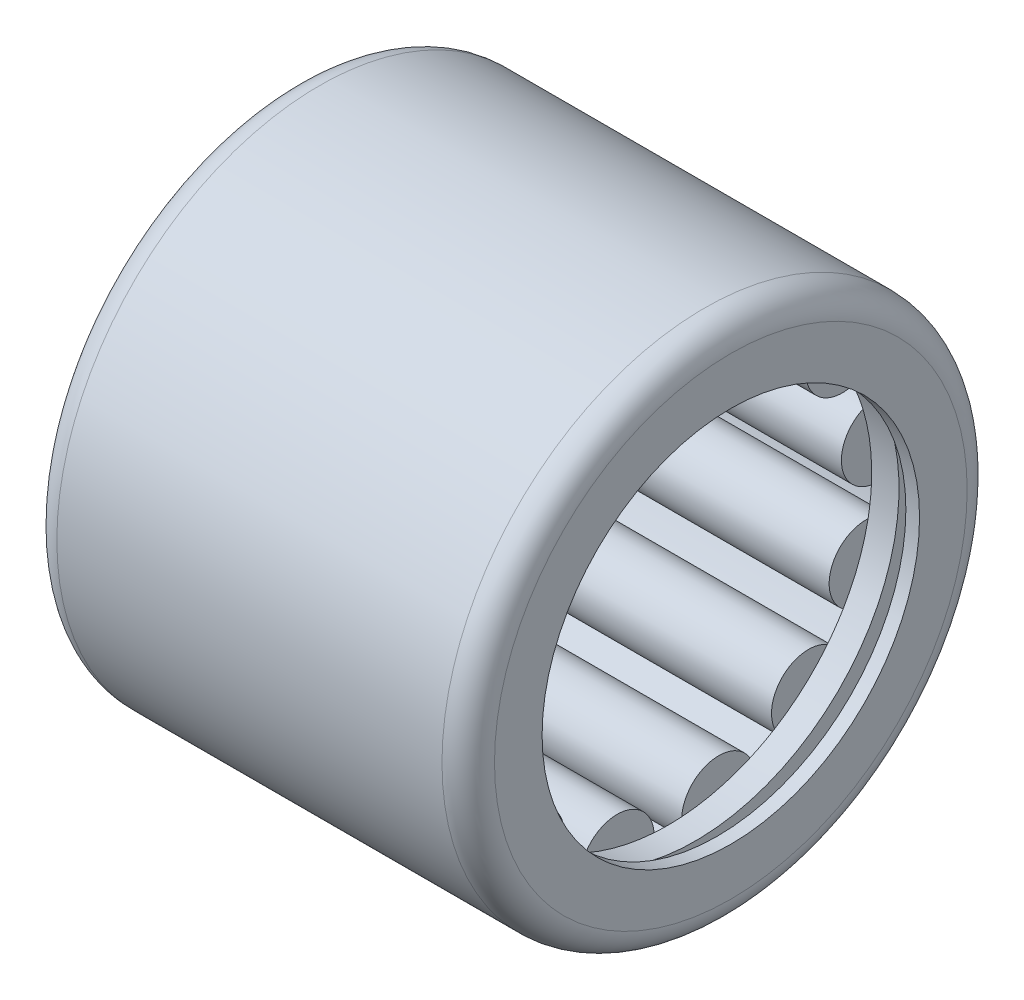
SolidWorks part; units mm, degrees
ref_plane "Front Plane" through (0, 0, 0) normal (0, 0, 1) x (1, 0, 0)
ref_plane "Top Plane" through (0, 0, 0) normal (0, 1, 0) x (1, 0, 0)
ref_plane "Right Plane" through (0, 0, 0) normal (1, 0, 0) x (0, 0, -1)
sketch "Dimension Sketch" plane through (0, 0, 0) normal (0, 0, 1) x (1, 0, 0)
  line L0 (0, 0) -> (12, 0)
  point P3 (8, 0)
  point P4 (10, 0)
  point P7 (0.6, 0)
sketch "Sketch1" plane through (0, 0, 0) normal (0, 0, 1) x (1, 0, 0)
  line L0 (0, 0) -> (3.6532, 0) construction
  line L1 (0, 0) -> (0, 6.2937) construction
  line L2 (0, 4) -> (10, 4)
  line L3 (0, 4.3125) -> (0, 6)
  line L4 (0, 6) -> (10, 6)
  line L5 (10, 4.3125) -> (10, 6)
  line L6 (0, 4.3125) -> (0.3125, 4.3125)
  line L7 (9.6875, 4.3125) -> (9.6875, 5.6875)
  line L8 (0.3125, 5.6875) -> (9.6875, 5.6875)
  line L9 (0.3125, 4.3125) -> (0.3125, 5.6875)
  line L10 (-4.6031, 4.8438) -> (23.1053, 4.8438) construction
  line L11 (9.6875, 4.3125) -> (10, 4.3125)
  line L12 (5, 6) -> (5, 4) construction
  line L13 (1.4375, 13) -> (1.4375, 10)
  line L14 (8.5625, 5.6875) -> (8.5625, 10)
  line L15 (1.4375, 13) -> (1.4375, 10)
  line L16 (8.5625, 13) -> (8.5625, 10)
  line L17 (1.125, 13) -> (1.125, 10)
  line L18 (8.875, 13) -> (8.875, 10)
  line L19 (0.8125, 13) -> (0.8125, 10)
  line L20 (9.1875, 5.6875) -> (9.1875, 4)
  line L21 (0.8125, 4.6562) -> (9.1875, 4.6562)
  line L22 (0.8125, 5.0312) -> (9.1875, 5.0312)
sketch "Sketch5" plane through (0, 0, 0) normal (0, 0, 1) x (1, 0, 0)
  line L1 (0.8125, 4.6562) -> (9.1875, 4.6562) construction
  line L2 (0.8125, 5.0312) -> (9.1875, 5.0312) construction
  line L3 (1.4375, 13) -> (1.4375, 10) construction
  line L4 (0.8125, 13) -> (0.8125, 10) construction
  line L6 (0.8125, 4.6562) -> (1.4375, 4.6562)
  line L7 (0.8125, 5.0312) -> (1.4375, 5.0312)
  line L8 (1.4375, 5.0312) -> (1.4375, 4.6562)
  line L9 (0.8125, 5.0312) -> (0.8125, 4.6562)
  line L14 (0, 0) -> (3.6532, 0) construction
  line L15 (0, 0) -> (3.6532, 0) construction
revolve "Base-Revolve2" add sketch "Sketch5" angle 360 about L15
sketch "Sketch6" plane through (0, 0, 0) normal (0, 0, 1) x (1, 0, 0)
  line L0 (-4.6031, 4.8438) -> (23.1053, 4.8438) construction
  line L4 (0.8125, 4.6562) -> (9.1875, 4.6562) construction
  line L5 (1.4375, 13) -> (1.4375, 10) construction
  line L6 (-4.6031, 4.8438) -> (23.1053, 4.8438) construction
  line L7 (1.125, 13) -> (1.125, 10) construction
  line L8 (1.125, 4.6562) -> (1.4375, 4.6562) construction
  line L9 (1.4375, 4.8438) -> (1.4375, 4.6562) construction
  line L10 (1.125, 4.8438) -> (1.125, 4.6562) construction
  line L11 (1.075, 4.8438) -> (1.075, 4.6063)
  line L12 (1.075, 4.6063) -> (1.4875, 4.6063)
  line L13 (1.4875, 4.8438) -> (1.4875, 4.6063)
  line L14 (1.075, 4.8438) -> (1.4875, 4.8438)
  dimension "D1" = 0.05
revolve "Cut-Revolve1" cut sketch "Sketch6" angle 360 about L6
pattern_circular "CirPattern3" count 13 over 360 about axis through (0, 0, 0) along (1, 0, 0) of "Cut-Revolve1"
sketch "Sketch3" plane through (0, 0, 0) normal (0, 0, 1) x (1, 0, 0)
  line L1 (0.3125, 5.6875) -> (9.6875, 5.6875) construction
  line L2 (8.5625, 5.6875) -> (8.5625, 10) construction
  line L3 (1.4375, 13) -> (1.4375, 10) construction
  line L4 (0.8125, 5.0312) -> (9.1875, 5.0312) construction
  line L6 (-4.6031, 4.8438) -> (23.1053, 4.8438) construction
  line L7 (1.4375, 5.6885) -> (8.5625, 5.6885)
  line L8 (2, 5.6875) -> (8.5625, 5.6875) construction
  line L9 (8.5625, 5.6885) -> (8.5625, 5.0312)
  line L10 (1.4375, 5.6885) -> (1.4375, 5.0312)
  line L11 (1.125, 5.0312) -> (1.4375, 5.0312)
  line L12 (8.875, 13) -> (8.875, 10) construction
  line L13 (-4.6031, 4.8438) -> (23.1053, 4.8438) construction
  line L14 (8.5625, 5.0312) -> (8.875, 5.0312)
  line L16 (1.125, 13) -> (1.125, 10) construction
  line L17 (8.875, 5.0312) -> (8.875, 4.8438)
  line L18 (1.125, 5.0312) -> (1.125, 4.8438)
  line L19 (1.125, 4.8438) -> (8.875, 4.8438)
  dimension "D1" = 0.001
revolve "Base-Revolve" add sketch "Sketch3" angle 360 about L13
sketch "Sketch2" plane through (0, 0, 0) normal (0, 0, 1) x (1, 0, 0)
  line L0 (0, 0) -> (3.6532, 0) construction
  line L1 (9.6875, 4.3125) -> (10, 4.3125) construction
  line L2 (0, 4.3125) -> (0.3125, 4.3125) construction
  line L3 (9.6875, 4.3125) -> (9.6875, 5.6875) construction
  line L4 (10, 4.3125) -> (10, 6) construction
  line L5 (0.3125, 5.6875) -> (9.6875, 5.6875) construction
  line L6 (0.3125, 4.3125) -> (0.3125, 5.6875) construction
  line L7 (0, 4.3125) -> (0, 6) construction
  line L8 (0, 6) -> (10, 6) construction
  line L9 (0, 0) -> (3.6532, 0) construction
  line L10 (9.6875, 4.3125) -> (10, 4.3125)
  line L11 (0, 4.3125) -> (0.3125, 4.3125)
  line L12 (9.6875, 4.3125) -> (9.6875, 5.6875)
  line L13 (10, 4.3125) -> (10, 6)
  line L14 (0.3125, 5.6875) -> (9.6875, 5.6875)
  line L15 (0.3125, 4.3125) -> (0.3125, 5.6875)
  line L16 (0, 4.3125) -> (0, 6)
  line L17 (0, 6) -> (10, 6)
revolve "Boss-Revolve2" add sketch "Sketch2" angle 360 about L9
ref_plane "Plane1" through (5, 0, 0) normal (-1, 0, 0) x (0, 0, 1)
mirror "Mirror1" about plane through (5, 0, 0) normal (-1, 0, 0) of "Base-Revolve2"
pattern_circular "CirPattern2" count 13 over 360 about axis through (0, 0, 0) along (1, 0, 0) of "Base-Revolve"
fillet "Fillet1" radius 0.6 2 edges at (0, 0, 6) (10, 0, 6)
mirror "Mirror2" about plane through (5, 0, 0) normal (-1, 0, 0) of "Base-Revolve"
equation "\"D3@Sketch1\" = \"D@Dimension Sketch\""
equation "\"D1@Sketch1\" = \"Fw@Dimension Sketch\""
equation "\"D2@Sketch1\" = \"C@Dimension Sketch\""
equation "\"D1@Fillet1\" = \"r@Dimension Sketch\""
equation "\"D4@Sketch1\" = \"D2@Sketch1\" / 32"
equation "\"D12@Sketch1\" =  ( \"D2@Sketch1\" - \"D4@Sketch1\" * 2 ) / 2 - 0.5 "
equation "\"D11@Sketch1\" = \"D12@Sketch1\""
equation "\"D8@Sketch1\" = \"D12@Sketch1\" - \"D4@Sketch1\" * 2"
equation "\"D7@Sketch1\" = \"D8@Sketch1\""
equation "\"D9@Sketch1\" = \"D4@Sketch1\"*1.2"
equation "\"D6@Sketch1\" = (  \"D8@Sketch1\" + \"D12@Sketch1\" )  / 2"
equation "\"D5@Sketch1\" = \"D6@Sketch1\""
equation "\"D1@CirPattern2\" = 3.14* ( \"D3@Sketch1\" / 2 - \"D4@Sketch1\" - \"D1@Sketch1\" / 2 )  * 2 /  ( \"D3@Sketch1\" - \"D1@Sketch1\" ) *5"
equation "\"D1@CirPattern3\" = \"D1@CirPattern2\""
